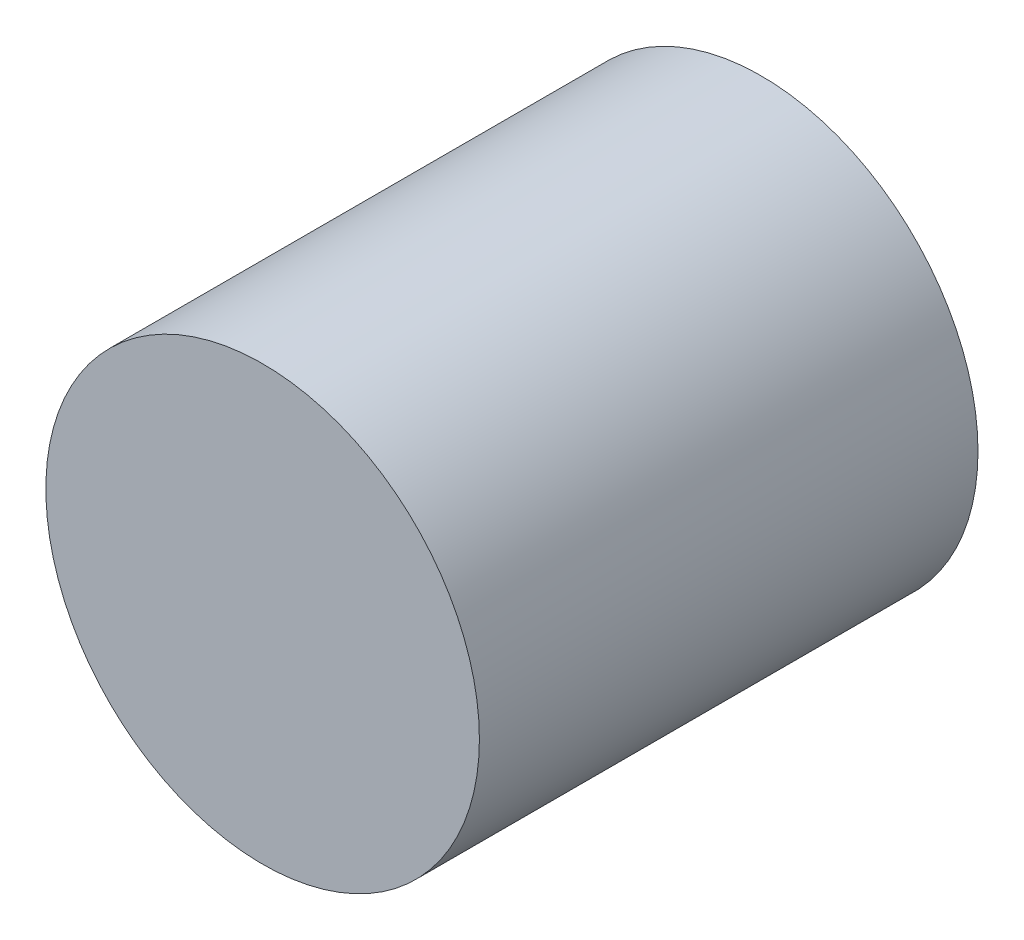
from build123d import *

# Parameters (mm, degrees)
SKETCH2_R           = 20
BOSS_EXTRUDE1_DEPTH = 46


with BuildPart() as part:
    # Sketch2 → Boss-Extrude1 (new body)
    with BuildSketch(Plane.XY):
        with Locations((121.674224319, 138.644018399)):
            Circle(SKETCH2_R)
    extrude(amount=BOSS_EXTRUDE1_DEPTH)


solid = part.part
